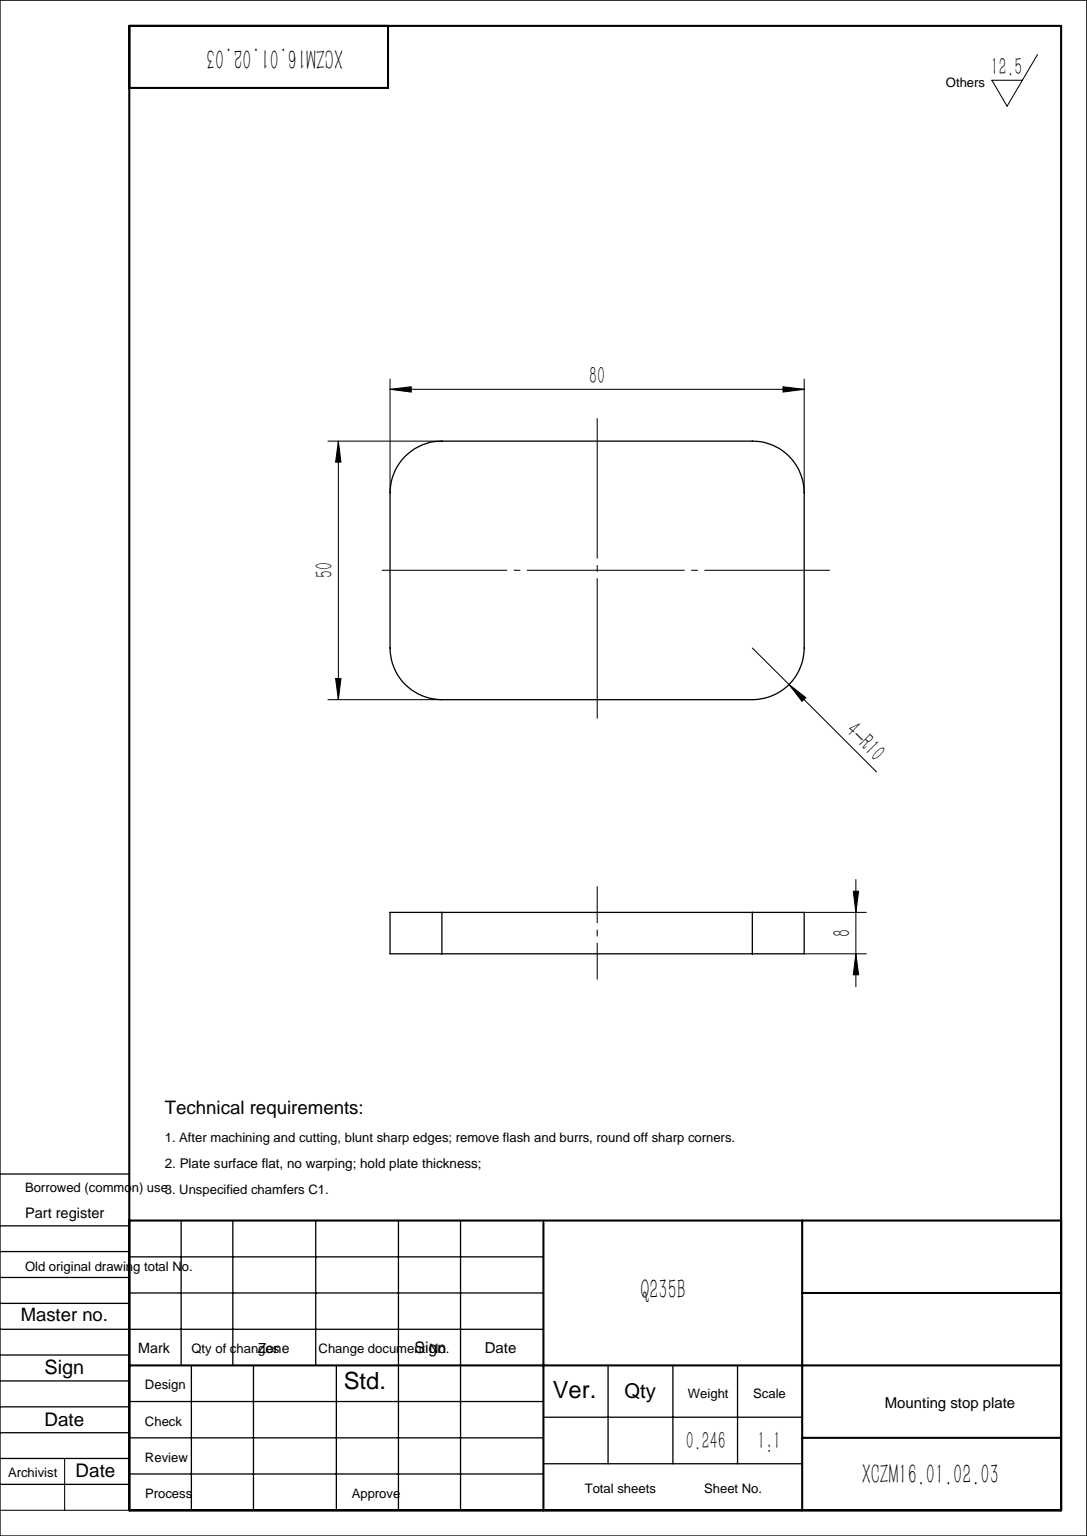
from build123d import *

# Parameters (mm, degrees)
BOSS_EXTRUDE1_DEPTH = 8


with BuildPart() as part:
    # Sketch1 → Boss-Extrude1 (new body)
    with BuildSketch(Plane.XY):
        with BuildLine():
            Line((30, -25), (-30, -25))
            ThreePointArc((-30, -25), (-37.071067812, -22.071067812), (-40, -15))
            Line((-40, -15), (-40, 15))
            ThreePointArc((-40, 15), (-37.071067812, 22.071067812), (-30, 25))
            Line((-30, 25), (30, 25))
            ThreePointArc((30, 25), (37.071067812, 22.071067812), (40, 15))
            Line((40, 15), (40, -15))
            ThreePointArc((40, -15), (37.071067812, -22.071067812), (30, -25))
        make_face()
    extrude(amount=BOSS_EXTRUDE1_DEPTH)


solid = part.part
